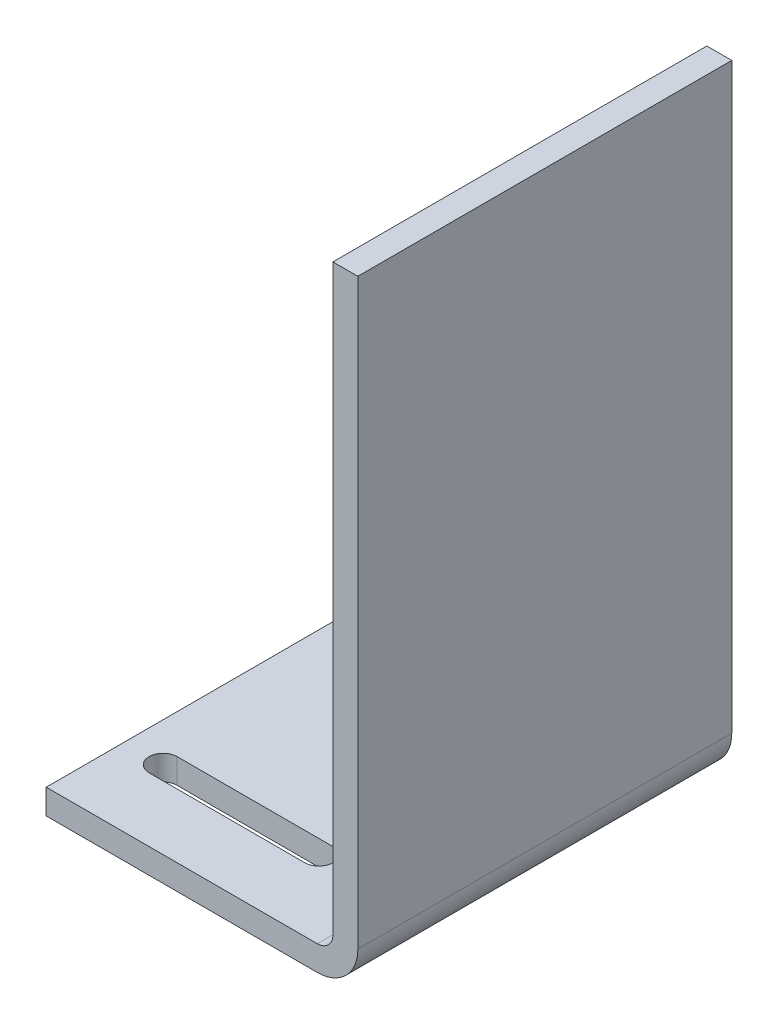
from build123d import *

# Parameters (mm, degrees)
BOSS_EXTRUDE1_DEPTH = 120
CUT_EXTRUDE1_DEPTH  = 120


with BuildPart() as part:
    # Sketch1 → Boss-Extrude1 (new body)
    with BuildSketch(Plane.XY):
        with BuildLine():
            Line((0, 0), (87, 0))
            ThreePointArc((87, 0), (96.192388155, 3.807611845), (100, 13))
            Line((100, 13), (100, 200))
            Line((100, 200), (92, 200))
            Line((92, 200), (92, 13))
            ThreePointArc((92, 13), (90.535533906, 9.464466094), (87, 8))
            Line((87, 8), (0, 8))
            Line((0, 8), (0, 0))
        make_face()
    extrude(amount=BOSS_EXTRUDE1_DEPTH)

    # Sketch2 → Cut-Extrude1 (cut)
    with BuildSketch(Plane(origin=(0, 8, 0), x_dir=(1, 0, 0), z_dir=(0, 1, 0))):
        with BuildLine():
            Line((12.5, -20.5), (62.5, -20.5))
            ThreePointArc((62.5, -20.5), (67, -25), (62.5, -29.5))
            Line((62.5, -29.5), (12.5, -29.5))
            ThreePointArc((12.5, -29.5), (8, -25), (12.5, -20.5))
        make_face()
        with BuildLine():
            Line((12.5, -99.5), (62.5, -99.5))
            ThreePointArc((62.5, -99.5), (67, -95), (62.5, -90.5))
            Line((62.5, -90.5), (12.5, -90.5))
            ThreePointArc((12.5, -90.5), (8, -95), (12.5, -99.5))
        make_face()
    extrude(amount=-CUT_EXTRUDE1_DEPTH, mode=Mode.SUBTRACT)


solid = part.part
